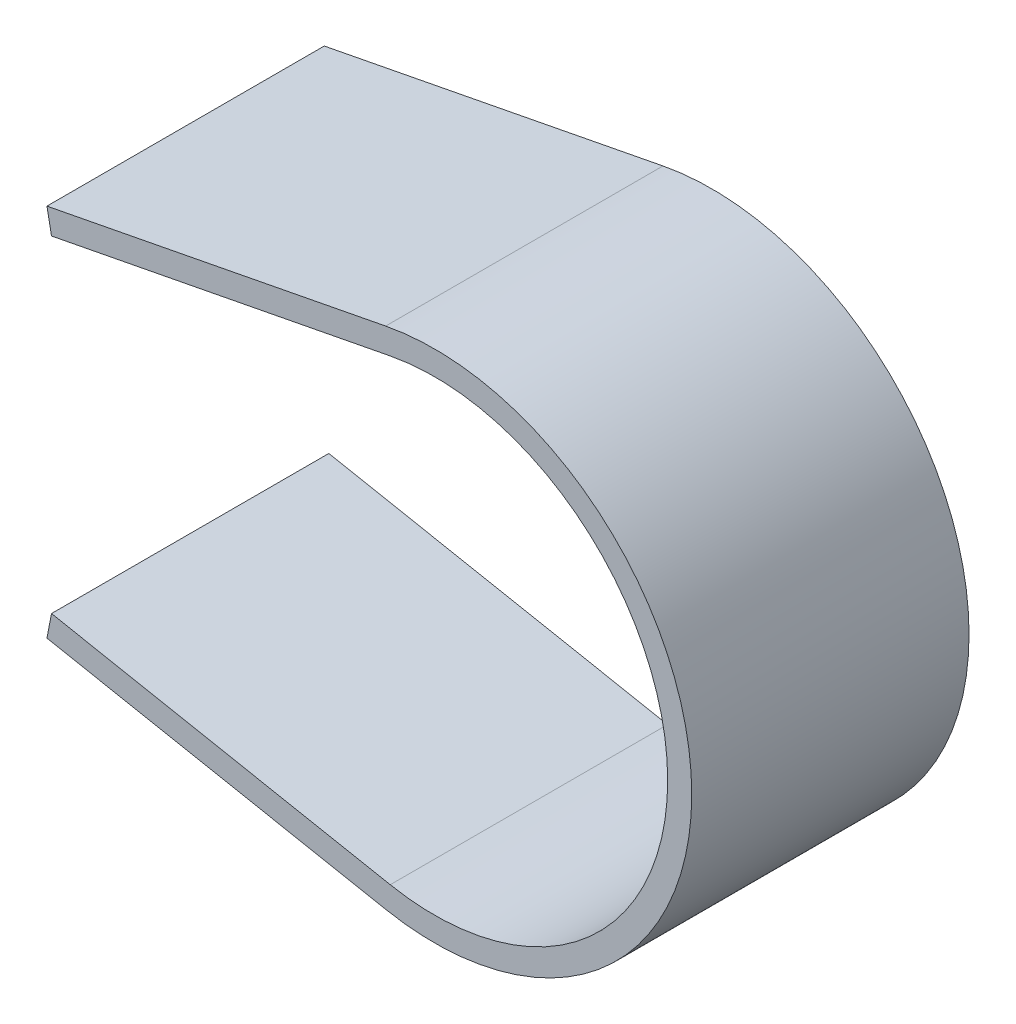
SolidWorks part; units mm, degrees
ref_plane "Front Plane" through (0, 0, 0) normal (0, 0, 1) x (1, 0, 0)
ref_plane "Top Plane" through (0, 0, 0) normal (0, 1, 0) x (1, 0, 0)
ref_plane "Right Plane" through (0, 0, 0) normal (1, 0, 0) x (0, 0, -1)
sketch "Sketch1" plane through (0, 0, 0) normal (0, 0, 1) x (1, 0, 0)
  line L0 (-290, 317.6106) -> (-290, -297.9308) construction
  line L1 (-290, 140) -> (-36.5386, 189.0005)
  line L2 (-290, -140) -> (-36.5386, -189.0005)
  line L3 (0, 0) -> (-450.9961, 0) construction
  line L4 (-286.5834, -122.3272) -> (-33.122, -171.3277)
  line L5 (-286.5834, 122.3272) -> (-33.122, 171.3277)
  line L6 (-290, 140) -> (-286.5834, 122.3272)
  line L7 (-286.5834, -122.3272) -> (-290, -140)
  arc A0 (-36.5386, -189.0005) -> (-36.5386, 189.0005) centre (0, 0) ccw
  arc A1 (-33.122, -171.3277) -> (-33.122, 171.3277) centre (0, 0) ccw
  dimension "D1" = 385
  dimension "D2" = 290
  dimension "D3" = 140
  dimension "D4" = 140
  dimension "D5" = 18
extrude "Boss-Extrude1" add sketch "Sketch1" along normal blind 207.5
